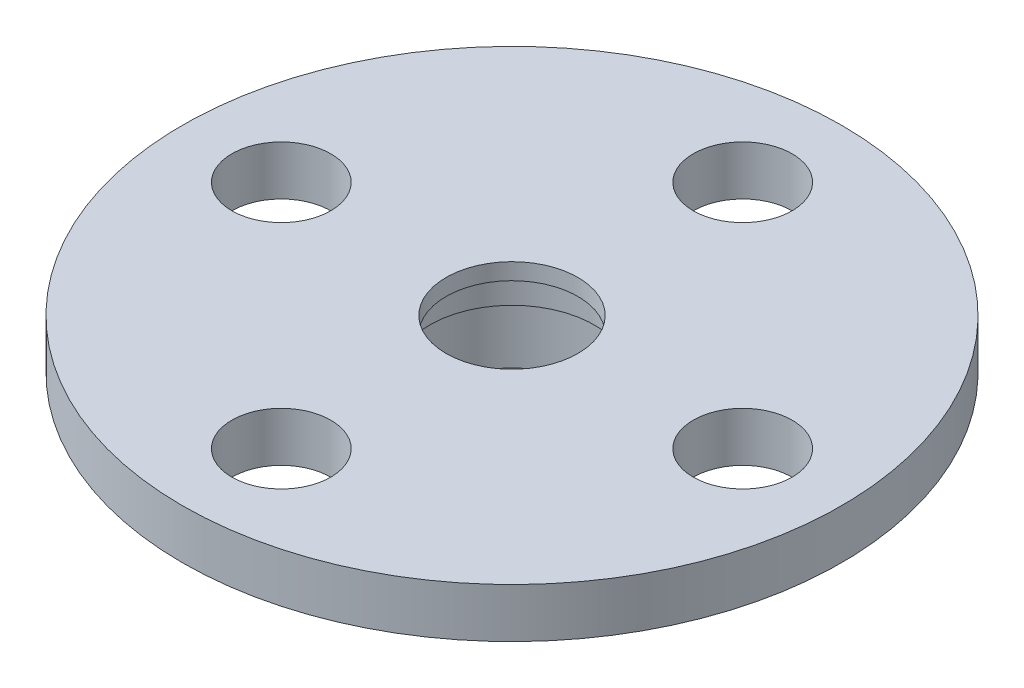
from build123d import *

# Parameters (mm, degrees)
SKETCH2_R          = 1.5
CUT_EXTRUDE1_DEPTH = 10


with BuildPart() as part:
    # Sketch1 → Revolve1 (revolve)
    with BuildSketch(Plane.XY, mode=Mode.PRIVATE) as revolve1_sk:
        Polygon((-0.138513514, 1.280405405), (7.861486486, 1.280405405), (7.861486486, -0.219594595), (1.861486486, -0.219594595), (1.861486486, -1.019594595), (1.861486486, -2.219594595), (0.861486486, -2.219594595), (0.861486486, -0.219594595), (0.361486486, -0.219594595), (0.361486486, 0.780405405), (-0.138513514, 0.780405405), align=None)
    revolve(revolve1_sk.sketch.rotate(Axis((-2.138513514, 1.540540541, 0), (0, -1, 0)), 90), axis=Axis((-2.138513514, 1.540540541, 0), (0, -1, 0)))

    # Sketch2 → Cut-Extrude1 (cut)
    with BuildSketch(Plane(origin=(0, 1.280405405, 0), x_dir=(1, 0, 0), z_dir=(0, 1, 0))):
        with Locations(Location((-2.138513514, 7, 0), (0, 0, 270))):
            Circle(SKETCH2_R)
        with Locations(Location((4.861486486, 0, 0), (0, 0, 270))):
            Circle(SKETCH2_R)
        with Locations(Location((-2.138513514, -7, 0), (0, 0, 269.999999999))):
            Circle(SKETCH2_R)
        with Locations(Location((-9.138513514, 0, 0), (0, 0, 270))):
            Circle(SKETCH2_R)
    extrude(amount=-CUT_EXTRUDE1_DEPTH, mode=Mode.SUBTRACT)


solid = part.part
